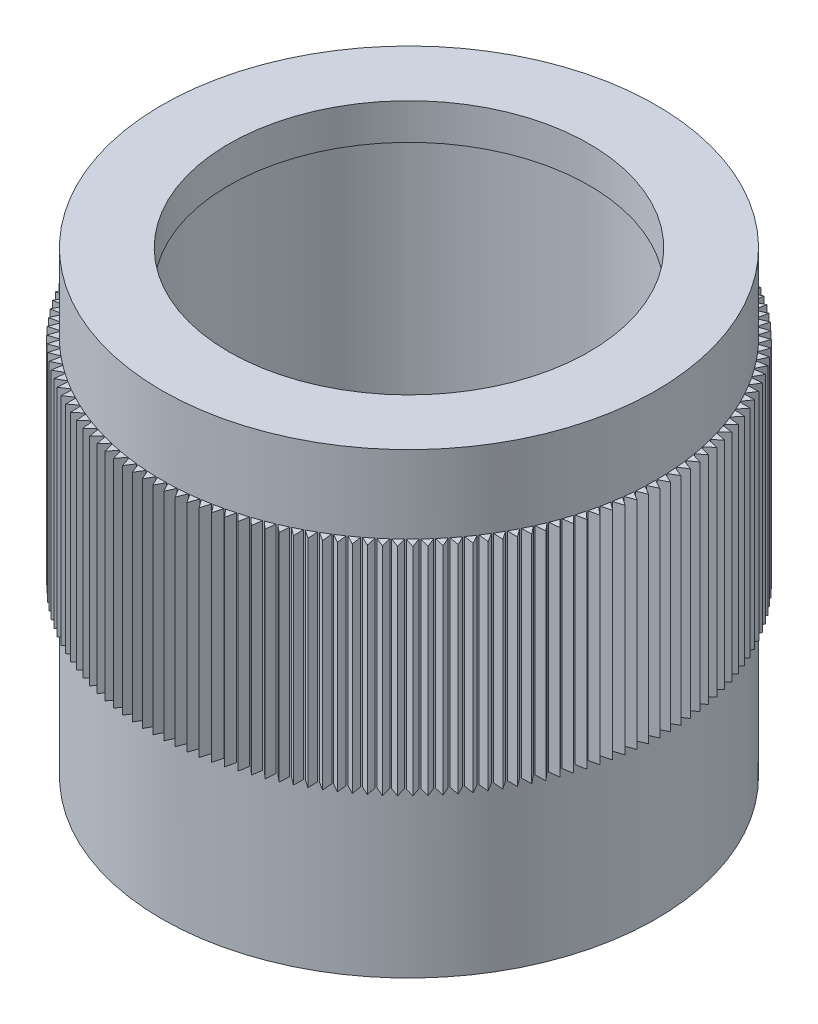
from build123d import *

# Parameters (mm, degrees)
BOSS_EXTRUDE1_DEPTH = 6
CHAMFER1_SIZE       = 0.5


with BuildPart() as part:
    # Sketch1 → Revolve1 (revolve)
    with BuildSketch(Plane.XY, mode=Mode.PRIVATE) as revolve1_sk:
        Polygon((-5, 11.7), (-5.25, 11.7), (-5.25, 0), (-6.86, 0), (-6.86, 12.7), (-5, 12.7), align=None)
    revolve(revolve1_sk.sketch.rotate(Axis((0, 15.254212557, 0), (0, -1, 0)), 270), axis=Axis((0, 15.254212557, 0), (0, -1, 0)))

    # Sketch2 → Boss-Extrude1 (add)
    with BuildSketch(Plane(origin=(0, 10.55, 0), x_dir=(-1, 0, 0), z_dir=(0, 1, 0))):
        with BuildLine():
            Line((-0.125, 6.858861057), (0, 7.11))
            Line((0, 7.11), (0.125, 6.858861057))
            ThreePointArc((0.125, 6.858861057), (0, 6.86), (-0.125, 6.858861057))
        make_face()
        with BuildLine():
            Line((0.162328937, 6.858079127), (0.297735898, 7.103763322))
            Line((0.297735898, 7.103763322), (0.412109644, 6.847610214))
            ThreePointArc((0.412109644, 6.847610214), (0.287266985, 6.853982614), (0.162328937, 6.858079127))
        make_face()
        with BuildLine():
            Line((0.449373094, 6.845265796), (0.594949466, 7.085064229))
            Line((0.594949466, 7.085064229), (0.698496308, 6.824346336))
            ThreePointArc((0.698496308, 6.824346336), (0.574030005, 6.835941014), (0.449373094, 6.845265796))
        make_face()
        with BuildLine():
            Line((0.735628897, 6.820443543), (0.891119291, 7.053935526))
            Line((0.891119291, 7.053935526), (0.983657573, 6.789110235))
            ThreePointArc((0.983657573, 6.789110235), (0.859785982, 6.805906851), (0.735628897, 6.820443543))
        make_face()
        with BuildLine():
            Line((1.020594158, 6.783655914), (1.185725789, 7.010431824))
            Line((1.185725789, 7.010431824), (1.267093167, 6.741963728))
            ThreePointArc((1.267093167, 6.741963728), (1.144033602, 6.763932814), (1.020594158, 6.783655914))
        make_face()
        with BuildLine():
            Line((1.303768949, 6.734967448), (1.478252122, 6.954629441))
            Line((1.478252122, 6.954629441), (1.54830585, 6.682989525))
            ThreePointArc((1.54830585, 6.682989525), (1.426274199, 6.710092541), (1.303768949, 6.734967448))
        make_face()
        with BuildLine():
            Line((1.584656487, 6.67446356), (1.768185098, 6.886626276))
            Line((1.768185098, 6.886626276), (1.826802277, 6.612291088))
            ThreePointArc((1.826802277, 6.612291088), (1.706012626, 6.644480485), (1.584656487, 6.67446356))
        make_face()
        with BuildLine():
            Line((1.862763999, 6.602250395), (2.055016076, 6.806541627))
            Line((2.055016076, 6.806541627), (2.102093874, 6.529992446))
            ThreePointArc((2.102093874, 6.529992446), (1.982758127, 6.567211753), (1.862763999, 6.602250395))
        make_face()
        with BuildLine():
            Line((2.13760359, 6.51845464), (2.338241858, 6.714515992))
            Line((2.338241858, 6.714515992), (2.373697683, 6.436237978))
            ThreePointArc((2.373697683, 6.436237978), (2.256025197, 6.4784219), (2.13760359, 6.51845464))
        make_face()
        with BuildLine():
            Line((2.408693098, 6.4232233), (2.61736557, 6.610710815))
            Line((2.61736557, 6.610710815), (2.641137219, 6.331192162))
            ThreePointArc((2.641137219, 6.331192162), (2.525334431, 6.378266693), (2.408693098, 6.4232233))
        make_face()
        with BuildLine():
            Line((2.675556939, 6.316723444), (2.891897532, 6.495308204))
            Line((2.891897532, 6.495308204), (2.903943304, 6.215039283))
            ThreePointArc((2.903943304, 6.215039283), (2.790213371, 6.266921839), (2.675556939, 6.316723444))
        make_face()
        with BuildLine():
            Line((2.937726945, 6.199141908), (3.161356124, 6.368510615))
            Line((3.161356124, 6.368510615), (3.161654885, 6.087983113))
            ThreePointArc((3.161654885, 6.087983113), (3.050197329, 6.144582675), (2.937726945, 6.199141908))
        make_face()
        with BuildLine():
            Line((3.194743179, 6.070684971), (3.425268623, 6.230540495))
            Line((3.425268623, 6.230540495), (3.413819849, 5.950246553))
            ThreePointArc((3.413819849, 5.950246553), (3.304830204, 6.011463825), (3.194743179, 6.070684971))
        make_face()
        with BuildLine():
            Line((3.446154749, 5.93157799), (3.683172037, 6.08163989))
            Line((3.683172037, 6.08163989), (3.659995814, 5.802071237))
            ThreePointArc((3.659995814, 5.802071237), (3.553665284, 5.867798825), (3.446154749, 5.93157799))
        make_face()
        with BuildLine():
            Line((3.691520591, 5.782065005), (3.934613915, 5.922070021))
            Line((3.934613915, 5.922070021), (3.899750901, 5.643717118))
            ThreePointArc((3.899750901, 5.643717118), (3.796266028, 5.713839711), (3.691520591, 5.782065005))
        make_face()
        with BuildLine():
            Line((3.930410253, 5.622408314), (4.179153144, 5.75211083))
            Line((4.179153144, 5.75211083), (4.132664501, 5.475462001))
            ThreePointArc((4.132664501, 5.475462001), (4.032206831, 5.549856581), (3.930410253, 5.622408314))
        make_face()
        with BuildLine():
            Line((4.162404639, 5.452888008), (4.416360718, 5.572060482))
            Line((4.416360718, 5.572060482), (4.358328003, 5.297601063))
            ThreePointArc((4.358328003, 5.297601063), (4.261073773, 5.376137117), (4.162404639, 5.452888008))
        make_face()
        with BuildLine():
            Line((4.387096753, 5.273801483), (4.645820494, 5.382234846))
            Line((4.645820494, 5.382234846), (4.576345517, 5.110446332))
            ThreePointArc((4.576345517, 5.110446332), (4.482465343, 5.192986082), (4.387096753, 5.273801483))
        make_face()
        with BuildLine():
            Line((4.604092408, 5.085462919), (4.867129923, 5.182966941))
            Line((4.867129923, 5.182966941), (4.786334565, 4.914326142))
            ThreePointArc((4.786334565, 4.914326142), (4.695993147, 5.000724784), (4.604092408, 5.085462919))
        make_face()
        with BuildLine():
            Line((4.813010921, 4.888202724), (5.079900752, 4.974606351))
            Line((5.079900752, 4.974606351), (4.987926756, 4.709584554))
            ThreePointArc((4.987926756, 4.709584554), (4.901282582, 4.799690516), (4.813010921, 4.888202724))
        make_face()
        with BuildLine():
            Line((5.013485777, 4.682366961), (5.283759709, 4.757518611))
            Line((5.283759709, 4.757518611), (5.180768429, 4.496580755))
            ThreePointArc((5.180768429, 4.496580755), (5.097973503, 4.59023596), (5.013485777, 4.682366961))
        make_face()
        with BuildLine():
            Line((5.205165276, 4.468316735), (5.478349156, 4.532084567))
            Line((5.478349156, 4.532084567), (5.364521274, 4.275688425))
            ThreePointArc((5.364521274, 4.275688425), (5.285720845, 4.37272857), (5.205165276, 4.468316735))
        make_face()
        with BuildLine():
            Line((5.387713146, 4.246427564), (5.663327717, 4.298699707))
            Line((5.663327717, 4.298699707), (5.538862925, 4.047295084))
            ThreePointArc((5.538862925, 4.047295084), (5.464195238, 4.147549928), (5.387713146, 4.246427564))
        make_face()
        with BuildLine():
            Line((5.560809137, 4.017088715), (5.838370877, 4.057773466))
            Line((5.838370877, 4.057773466), (5.703487529, 3.811801413))
            ThreePointArc((5.703487529, 3.811801413), (5.633083575, 3.915095074), (5.560809137, 4.017088715))
        make_face()
        with BuildLine():
            Line((5.724149578, 3.780702528), (6.00317155, 3.809728512))
            Line((6.00317155, 3.809728512), (5.858106277, 3.569620547))
            ThreePointArc((5.858106277, 3.569620547), (5.792089569, 3.675771814), (5.724149578, 3.780702528))
        make_face()
        with BuildLine():
            Line((5.877447916, 3.537683704), (6.157440621, 3.555))
            Line((6.157440621, 3.555), (6.002447916, 3.321177353))
            ThreePointArc((6.002447916, 3.321177353), (5.94093427, 3.43), (5.877447916, 3.537683704))
        make_face()
        with BuildLine():
            Line((6.020435214, 3.288458581), (6.300907448, 3.29403481))
            Line((6.300907448, 3.29403481), (6.136259223, 3.066907686))
            ThreePointArc((6.136259223, 3.066907686), (6.079356554, 3.178210801), (6.020435214, 3.288458581))
        make_face()
        with BuildLine():
            Line((6.152860622, 3.033464383), (6.433320343, 3.027290763))
            Line((6.433320343, 3.027290763), (6.259305445, 2.80725762))
            ThreePointArc((6.259305445, 2.80725762), (6.20711358, 2.92084594), (6.152860622, 3.033464383))
        make_face()
        with BuildLine():
            Line((6.274491822, 2.773148459), (6.554447008, 2.75523582))
            Line((6.554447008, 2.75523582), (6.371370719, 2.542682671))
            ThreePointArc((6.371370719, 2.542682671), (6.32398122, 2.658356923), (6.274491822, 2.773148459))
        make_face()
        with BuildLine():
            Line((6.385115431, 2.50796749), (6.664074945, 2.478347256))
            Line((6.664074945, 2.478347256), (6.472258443, 2.273646992))
            ThreePointArc((6.472258443, 2.273646992), (6.429754448, 2.391204245), (6.385115431, 2.50796749))
        make_face()
        with BuildLine():
            Line((6.484537378, 2.238386693), (6.762011831, 2.19711083))
            Line((6.762011831, 2.19711083), (6.561791627, 2.000622564))
            ThreePointArc((6.561791627, 2.000622564), (6.524247702, 2.119856581), (6.484537378, 2.238386693))
        make_face()
        with BuildLine():
            Line((6.572583243, 1.964879006), (6.84808585, 1.912019925))
            Line((6.84808585, 1.912019925), (6.639813199, 1.724088364))
            ThreePointArc((6.639813199, 1.724088364), (6.607295208, 1.844789969), (6.572583243, 1.964879006))
        make_face()
        with BuildLine():
            Line((6.649098564, 1.687924253), (6.922145999, 1.623574686))
            Line((6.922145999, 1.623574686), (6.706186282, 1.444529527))
            ThreePointArc((6.706186282, 1.444529527), (6.678751274, 1.566486969), (6.649098564, 1.687924253))
        make_face()
        with BuildLine():
            Line((6.713949107, 1.408008308), (6.984062353, 1.332281147))
            Line((6.984062353, 1.332281147), (6.760794435, 1.162436495))
            ThreePointArc((6.760794435, 1.162436495), (6.73849054, 1.285435818), (6.713949107, 1.408008308))
        make_face()
        with BuildLine():
            Line((6.767021101, 1.125622237), (7.033726287, 1.038650333))
            Line((7.033726287, 1.038650333), (6.803541858, 0.878304154))
            ThreePointArc((6.803541858, 0.878304154), (6.786408204, 1.002129576), (6.767021101, 1.125622237))
        make_face()
        with BuildLine():
            Line((6.808221441, 0.841261443), (7.071050676, 0.743197374))
            Line((7.071050676, 0.743197374), (6.834353556, 0.592630969))
            ThreePointArc((6.834353556, 0.592630969), (6.822420202, 0.717065258), (6.808221441, 0.841261443))
        make_face()
        with BuildLine():
            Line((6.837477847, 0.55542479), (7.095970039, 0.446440594))
            Line((7.095970039, 0.446440594), (6.853175476, 0.305918108))
            ThreePointArc((6.853175476, 0.305918108), (6.846463357, 0.430742964), (6.837477847, 0.55542479))
        make_face()
        with BuildLine():
            Line((6.854738993, 0.268613734), (7.10844066, 0.148900605))
            Line((7.10844066, 0.148900605), (6.859974598, 0.018668563))
            ThreePointArc((6.859974598, 0.018668563), (6.858495489, 0.143665), (6.854738993, 0.268613734))
        make_face()
        with BuildLine():
            Line((6.859974598, -0.018668563), (7.10844066, -0.148900605))
            Line((7.10844066, -0.148900605), (6.854738993, -0.268613734))
            ThreePointArc((6.854738993, -0.268613734), (6.858495489, -0.143665), (6.859974598, -0.018668563))
        make_face()
        with BuildLine():
            Line((6.853175476, -0.305918108), (7.095970039, -0.446440594))
            Line((7.095970039, -0.446440594), (6.837477847, -0.55542479))
            ThreePointArc((6.837477847, -0.55542479), (6.846463357, -0.430742964), (6.853175476, -0.305918108))
        make_face()
        with BuildLine():
            Line((6.834353556, -0.592630969), (7.071050676, -0.743197374))
            Line((7.071050676, -0.743197374), (6.808221441, -0.841261443))
            ThreePointArc((6.808221441, -0.841261443), (6.822420202, -0.717065258), (6.834353556, -0.592630969))
        make_face()
        with BuildLine():
            Line((6.803541858, -0.878304154), (7.033726287, -1.038650333))
            Line((7.033726287, -1.038650333), (6.767021101, -1.125622237))
            ThreePointArc((6.767021101, -1.125622237), (6.786408204, -1.002129576), (6.803541858, -0.878304154))
        make_face()
        with BuildLine():
            Line((6.760794435, -1.162436495), (6.984062353, -1.332281147))
            Line((6.984062353, -1.332281147), (6.713949107, -1.408008308))
            ThreePointArc((6.713949107, -1.408008308), (6.73849054, -1.285435818), (6.760794435, -1.162436495))
        make_face()
        with BuildLine():
            Line((6.706186282, -1.444529527), (6.922145999, -1.623574686))
            Line((6.922145999, -1.623574686), (6.649098564, -1.687924253))
            ThreePointArc((6.649098564, -1.687924253), (6.678751274, -1.566486969), (6.706186282, -1.444529527))
        make_face()
        with BuildLine():
            Line((6.639813199, -1.724088364), (6.84808585, -1.912019925))
            Line((6.84808585, -1.912019925), (6.572583243, -1.964879006))
            ThreePointArc((6.572583243, -1.964879006), (6.607295208, -1.844789969), (6.639813199, -1.724088364))
        make_face()
        with BuildLine():
            Line((6.561791627, -2.000622564), (6.762011831, -2.19711083))
            Line((6.762011831, -2.19711083), (6.484537378, -2.238386693))
            ThreePointArc((6.484537378, -2.238386693), (6.524247702, -2.119856581), (6.561791627, -2.000622564))
        make_face()
        with BuildLine():
            Line((6.472258443, -2.273646992), (6.664074945, -2.478347256))
            Line((6.664074945, -2.478347256), (6.385115431, -2.50796749))
            ThreePointArc((6.385115431, -2.50796749), (6.429754448, -2.391204245), (6.472258443, -2.273646992))
        make_face()
        with BuildLine():
            Line((6.371370719, -2.542682671), (6.554447008, -2.75523582))
            Line((6.554447008, -2.75523582), (6.274491822, -2.773148459))
            ThreePointArc((6.274491822, -2.773148459), (6.32398122, -2.658356923), (6.371370719, -2.542682671))
        make_face()
        with BuildLine():
            Line((6.259305445, -2.80725762), (6.433320343, -3.027290763))
            Line((6.433320343, -3.027290763), (6.152860622, -3.033464383))
            ThreePointArc((6.152860622, -3.033464383), (6.20711358, -2.92084594), (6.259305445, -2.80725762))
        make_face()
        with BuildLine():
            Line((6.136259223, -3.066907686), (6.300907448, -3.29403481))
            Line((6.300907448, -3.29403481), (6.020435214, -3.288458581))
            ThreePointArc((6.020435214, -3.288458581), (6.079356554, -3.178210801), (6.136259223, -3.066907686))
        make_face()
        with BuildLine():
            Line((6.002447916, -3.321177353), (6.157440621, -3.555))
            Line((6.157440621, -3.555), (5.877447916, -3.537683704))
            ThreePointArc((5.877447916, -3.537683704), (5.94093427, -3.43), (6.002447916, -3.321177353))
        make_face()
        with BuildLine():
            Line((5.858106277, -3.569620547), (6.00317155, -3.809728512))
            Line((6.00317155, -3.809728512), (5.724149578, -3.780702528))
            ThreePointArc((5.724149578, -3.780702528), (5.792089569, -3.675771814), (5.858106277, -3.569620547))
        make_face()
        with BuildLine():
            Line((5.703487529, -3.811801413), (5.838370877, -4.057773466))
            Line((5.838370877, -4.057773466), (5.560809137, -4.017088715))
            ThreePointArc((5.560809137, -4.017088715), (5.633083575, -3.915095074), (5.703487529, -3.811801413))
        make_face()
        with BuildLine():
            Line((5.538862925, -4.047295084), (5.663327717, -4.298699707))
            Line((5.663327717, -4.298699707), (5.387713146, -4.246427564))
            ThreePointArc((5.387713146, -4.246427564), (5.464195238, -4.147549928), (5.538862925, -4.047295084))
        make_face()
        with BuildLine():
            Line((5.364521274, -4.275688425), (5.478349156, -4.532084567))
            Line((5.478349156, -4.532084567), (5.205165276, -4.468316735))
            ThreePointArc((5.205165276, -4.468316735), (5.285720845, -4.37272857), (5.364521274, -4.275688425))
        make_face()
        with BuildLine():
            Line((5.180768429, -4.496580755), (5.283759709, -4.757518611))
            Line((5.283759709, -4.757518611), (5.013485777, -4.682366961))
            ThreePointArc((5.013485777, -4.682366961), (5.097973503, -4.59023596), (5.180768429, -4.496580755))
        make_face()
        with BuildLine():
            Line((4.987926756, -4.709584554), (5.079900752, -4.974606351))
            Line((5.079900752, -4.974606351), (4.813010921, -4.888202724))
            ThreePointArc((4.813010921, -4.888202724), (4.901282582, -4.799690516), (4.987926756, -4.709584554))
        make_face()
        with BuildLine():
            Line((4.786334565, -4.914326142), (4.867129923, -5.182966941))
            Line((4.867129923, -5.182966941), (4.604092408, -5.085462919))
            ThreePointArc((4.604092408, -5.085462919), (4.695993147, -5.000724784), (4.786334565, -4.914326142))
        make_face()
        with BuildLine():
            Line((4.576345517, -5.110446332), (4.645820494, -5.382234846))
            Line((4.645820494, -5.382234846), (4.387096753, -5.273801483))
            ThreePointArc((4.387096753, -5.273801483), (4.482465343, -5.192986082), (4.576345517, -5.110446332))
        make_face()
        with BuildLine():
            Line((4.358328003, -5.297601063), (4.416360718, -5.572060482))
            Line((4.416360718, -5.572060482), (4.162404639, -5.452888008))
            ThreePointArc((4.162404639, -5.452888008), (4.261073773, -5.376137117), (4.358328003, -5.297601063))
        make_face()
        with BuildLine():
            Line((4.132664501, -5.475462001), (4.179153144, -5.75211083))
            Line((4.179153144, -5.75211083), (3.930410253, -5.622408314))
            ThreePointArc((3.930410253, -5.622408314), (4.032206831, -5.549856581), (4.132664501, -5.475462001))
        make_face()
        with BuildLine():
            Line((3.899750901, -5.643717118), (3.934613915, -5.922070021))
            Line((3.934613915, -5.922070021), (3.691520591, -5.782065005))
            ThreePointArc((3.691520591, -5.782065005), (3.796266028, -5.713839711), (3.899750901, -5.643717118))
        make_face()
        with BuildLine():
            Line((3.659995814, -5.802071237), (3.683172037, -6.08163989))
            Line((3.683172037, -6.08163989), (3.446154749, -5.93157799))
            ThreePointArc((3.446154749, -5.93157799), (3.553665284, -5.867798825), (3.659995814, -5.802071237))
        make_face()
        with BuildLine():
            Line((3.413819849, -5.950246553), (3.425268623, -6.230540495))
            Line((3.425268623, -6.230540495), (3.194743179, -6.070684971))
            ThreePointArc((3.194743179, -6.070684971), (3.304830204, -6.011463825), (3.413819849, -5.950246553))
        make_face()
        with BuildLine():
            Line((3.161654885, -6.087983113), (3.161356124, -6.368510615))
            Line((3.161356124, -6.368510615), (2.937726945, -6.199141908))
            ThreePointArc((2.937726945, -6.199141908), (3.050197329, -6.144582675), (3.161654885, -6.087983113))
        make_face()
        with BuildLine():
            Line((2.903943304, -6.215039283), (2.891897532, -6.495308204))
            Line((2.891897532, -6.495308204), (2.675556939, -6.316723444))
            ThreePointArc((2.675556939, -6.316723444), (2.790213372, -6.266921839), (2.903943304, -6.215039283))
        make_face()
        with BuildLine():
            Line((2.641137219, -6.331192162), (2.61736557, -6.610710815))
            Line((2.61736557, -6.610710815), (2.408693098, -6.4232233))
            ThreePointArc((2.408693098, -6.4232233), (2.525334431, -6.378266693), (2.641137219, -6.331192162))
        make_face()
        with BuildLine():
            Line((2.373697683, -6.436237978), (2.338241858, -6.714515992))
            Line((2.338241858, -6.714515992), (2.13760359, -6.51845464))
            ThreePointArc((2.13760359, -6.51845464), (2.256025197, -6.4784219), (2.373697683, -6.436237978))
        make_face()
        with BuildLine():
            Line((2.102093874, -6.529992446), (2.055016076, -6.806541627))
            Line((2.055016076, -6.806541627), (1.862763999, -6.602250395))
            ThreePointArc((1.862763999, -6.602250395), (1.982758127, -6.567211753), (2.102093874, -6.529992446))
        make_face()
        with BuildLine():
            Line((1.826802277, -6.612291088), (1.768185098, -6.886626276))
            Line((1.768185098, -6.886626276), (1.584656487, -6.67446356))
            ThreePointArc((1.584656487, -6.67446356), (1.706012626, -6.644480485), (1.826802277, -6.612291088))
        make_face()
        with BuildLine():
            Line((1.54830585, -6.682989525), (1.478252122, -6.954629441))
            Line((1.478252122, -6.954629441), (1.303768949, -6.734967448))
            ThreePointArc((1.303768949, -6.734967448), (1.426274199, -6.710092541), (1.54830585, -6.682989525))
        make_face()
        with BuildLine():
            Line((1.267093167, -6.741963728), (1.185725789, -7.010431824))
            Line((1.185725789, -7.010431824), (1.020594158, -6.783655914))
            ThreePointArc((1.020594158, -6.783655914), (1.144033602, -6.763932814), (1.267093167, -6.741963728))
        make_face()
        with BuildLine():
            Line((0.983657573, -6.789110235), (0.891119291, -7.053935526))
            Line((0.891119291, -7.053935526), (0.735628897, -6.820443543))
            ThreePointArc((0.735628897, -6.820443543), (0.859785982, -6.805906851), (0.983657573, -6.789110235))
        make_face()
        with BuildLine():
            Line((0.698496308, -6.824346336), (0.594949466, -7.085064229))
            Line((0.594949466, -7.085064229), (0.449373094, -6.845265796))
            ThreePointArc((0.449373094, -6.845265796), (0.574030005, -6.835941014), (0.698496308, -6.824346336))
        make_face()
        with BuildLine():
            Line((0.412109644, -6.847610214), (0.297735898, -7.103763322))
            Line((0.297735898, -7.103763322), (0.162328937, -6.858079127))
            ThreePointArc((0.162328937, -6.858079127), (0.287266985, -6.853982614), (0.412109644, -6.847610214))
        make_face()
        with BuildLine():
            Line((0.125, -6.858861057), (0, -7.11))
            Line((0, -7.11), (-0.125, -6.858861057))
            ThreePointArc((-0.125, -6.858861057), (0, -6.86), (0.125, -6.858861057))
        make_face()
        with BuildLine():
            Line((-0.162328937, -6.858079127), (-0.297735898, -7.103763322))
            Line((-0.297735898, -7.103763322), (-0.412109644, -6.847610214))
            ThreePointArc((-0.412109644, -6.847610214), (-0.287266985, -6.853982614), (-0.162328937, -6.858079127))
        make_face()
        with BuildLine():
            Line((-0.449373094, -6.845265796), (-0.594949466, -7.085064229))
            Line((-0.594949466, -7.085064229), (-0.698496308, -6.824346336))
            ThreePointArc((-0.698496308, -6.824346336), (-0.574030005, -6.835941014), (-0.449373094, -6.845265796))
        make_face()
        with BuildLine():
            Line((-0.735628897, -6.820443543), (-0.891119291, -7.053935526))
            Line((-0.891119291, -7.053935526), (-0.983657573, -6.789110235))
            ThreePointArc((-0.983657573, -6.789110235), (-0.859785982, -6.805906851), (-0.735628897, -6.820443543))
        make_face()
        with BuildLine():
            Line((-1.020594158, -6.783655914), (-1.185725789, -7.010431824))
            Line((-1.185725789, -7.010431824), (-1.267093167, -6.741963728))
            ThreePointArc((-1.267093167, -6.741963728), (-1.144033602, -6.763932814), (-1.020594158, -6.783655914))
        make_face()
        with BuildLine():
            Line((-1.303768949, -6.734967448), (-1.478252122, -6.954629441))
            Line((-1.478252122, -6.954629441), (-1.54830585, -6.682989525))
            ThreePointArc((-1.54830585, -6.682989525), (-1.426274199, -6.710092541), (-1.303768949, -6.734967448))
        make_face()
        with BuildLine():
            Line((-1.584656487, -6.67446356), (-1.768185098, -6.886626276))
            Line((-1.768185098, -6.886626276), (-1.826802277, -6.612291088))
            ThreePointArc((-1.826802277, -6.612291088), (-1.706012626, -6.644480485), (-1.584656487, -6.67446356))
        make_face()
        with BuildLine():
            Line((-1.862763999, -6.602250395), (-2.055016076, -6.806541627))
            Line((-2.055016076, -6.806541627), (-2.102093874, -6.529992446))
            ThreePointArc((-2.102093874, -6.529992446), (-1.982758127, -6.567211753), (-1.862763999, -6.602250395))
        make_face()
        with BuildLine():
            Line((-2.13760359, -6.51845464), (-2.338241858, -6.714515992))
            Line((-2.338241858, -6.714515992), (-2.373697683, -6.436237978))
            ThreePointArc((-2.373697683, -6.436237978), (-2.256025197, -6.4784219), (-2.13760359, -6.51845464))
        make_face()
        with BuildLine():
            Line((-2.408693098, -6.4232233), (-2.61736557, -6.610710815))
            Line((-2.61736557, -6.610710815), (-2.641137219, -6.331192162))
            ThreePointArc((-2.641137219, -6.331192162), (-2.525334431, -6.378266693), (-2.408693098, -6.4232233))
        make_face()
        with BuildLine():
            Line((-2.675556939, -6.316723444), (-2.891897532, -6.495308204))
            Line((-2.891897532, -6.495308204), (-2.903943304, -6.215039283))
            ThreePointArc((-2.903943304, -6.215039283), (-2.790213371, -6.266921839), (-2.675556939, -6.316723444))
        make_face()
        with BuildLine():
            Line((-2.937726945, -6.199141908), (-3.161356124, -6.368510615))
            Line((-3.161356124, -6.368510615), (-3.161654885, -6.087983113))
            ThreePointArc((-3.161654885, -6.087983113), (-3.050197329, -6.144582675), (-2.937726945, -6.199141908))
        make_face()
        with BuildLine():
            Line((-3.194743179, -6.070684971), (-3.425268623, -6.230540495))
            Line((-3.425268623, -6.230540495), (-3.413819849, -5.950246553))
            ThreePointArc((-3.413819849, -5.950246553), (-3.304830204, -6.011463825), (-3.194743179, -6.070684971))
        make_face()
        with BuildLine():
            Line((-3.446154749, -5.93157799), (-3.683172037, -6.08163989))
            Line((-3.683172037, -6.08163989), (-3.659995814, -5.802071237))
            ThreePointArc((-3.659995814, -5.802071237), (-3.553665284, -5.867798825), (-3.446154749, -5.93157799))
        make_face()
        with BuildLine():
            Line((-3.691520591, -5.782065005), (-3.934613915, -5.922070021))
            Line((-3.934613915, -5.922070021), (-3.899750901, -5.643717118))
            ThreePointArc((-3.899750901, -5.643717118), (-3.796266028, -5.713839711), (-3.691520591, -5.782065005))
        make_face()
        with BuildLine():
            Line((-3.930410253, -5.622408314), (-4.179153144, -5.75211083))
            Line((-4.179153144, -5.75211083), (-4.132664501, -5.475462001))
            ThreePointArc((-4.132664501, -5.475462001), (-4.032206831, -5.549856581), (-3.930410253, -5.622408314))
        make_face()
        with BuildLine():
            Line((-4.162404639, -5.452888008), (-4.416360718, -5.572060482))
            Line((-4.416360718, -5.572060482), (-4.358328003, -5.297601063))
            ThreePointArc((-4.358328003, -5.297601063), (-4.261073773, -5.376137117), (-4.162404639, -5.452888008))
        make_face()
        with BuildLine():
            Line((-4.387096753, -5.273801483), (-4.645820494, -5.382234846))
            Line((-4.645820494, -5.382234846), (-4.576345517, -5.110446332))
            ThreePointArc((-4.576345517, -5.110446332), (-4.482465343, -5.192986082), (-4.387096753, -5.273801483))
        make_face()
        with BuildLine():
            Line((-4.604092408, -5.085462919), (-4.867129923, -5.182966941))
            Line((-4.867129923, -5.182966941), (-4.786334565, -4.914326142))
            ThreePointArc((-4.786334565, -4.914326142), (-4.695993147, -5.000724784), (-4.604092408, -5.085462919))
        make_face()
        with BuildLine():
            Line((-4.813010921, -4.888202724), (-5.079900752, -4.974606351))
            Line((-5.079900752, -4.974606351), (-4.987926756, -4.709584554))
            ThreePointArc((-4.987926756, -4.709584554), (-4.901282582, -4.799690516), (-4.813010921, -4.888202724))
        make_face()
        with BuildLine():
            Line((-5.013485777, -4.682366961), (-5.283759709, -4.757518611))
            Line((-5.283759709, -4.757518611), (-5.180768429, -4.496580755))
            ThreePointArc((-5.180768429, -4.496580755), (-5.097973503, -4.59023596), (-5.013485777, -4.682366961))
        make_face()
        with BuildLine():
            Line((-5.205165276, -4.468316735), (-5.478349156, -4.532084567))
            Line((-5.478349156, -4.532084567), (-5.364521274, -4.275688425))
            ThreePointArc((-5.364521274, -4.275688425), (-5.285720845, -4.37272857), (-5.205165276, -4.468316735))
        make_face()
        with BuildLine():
            Line((-5.387713146, -4.246427564), (-5.663327717, -4.298699707))
            Line((-5.663327717, -4.298699707), (-5.538862925, -4.047295084))
            ThreePointArc((-5.538862925, -4.047295084), (-5.464195238, -4.147549928), (-5.387713146, -4.246427564))
        make_face()
        with BuildLine():
            Line((-5.560809137, -4.017088715), (-5.838370877, -4.057773466))
            Line((-5.838370877, -4.057773466), (-5.703487529, -3.811801413))
            ThreePointArc((-5.703487529, -3.811801413), (-5.633083575, -3.915095074), (-5.560809137, -4.017088715))
        make_face()
        with BuildLine():
            Line((-5.724149578, -3.780702528), (-6.00317155, -3.809728512))
            Line((-6.00317155, -3.809728512), (-5.858106277, -3.569620547))
            ThreePointArc((-5.858106277, -3.569620547), (-5.792089569, -3.675771814), (-5.724149578, -3.780702528))
        make_face()
        with BuildLine():
            Line((-5.877447916, -3.537683704), (-6.157440621, -3.555))
            Line((-6.157440621, -3.555), (-6.002447916, -3.321177353))
            ThreePointArc((-6.002447916, -3.321177353), (-5.94093427, -3.43), (-5.877447916, -3.537683704))
        make_face()
        with BuildLine():
            Line((-6.020435214, -3.288458581), (-6.300907448, -3.29403481))
            Line((-6.300907448, -3.29403481), (-6.136259223, -3.066907686))
            ThreePointArc((-6.136259223, -3.066907686), (-6.079356554, -3.178210801), (-6.020435214, -3.288458581))
        make_face()
        with BuildLine():
            Line((-6.152860622, -3.033464383), (-6.433320343, -3.027290763))
            Line((-6.433320343, -3.027290763), (-6.259305445, -2.80725762))
            ThreePointArc((-6.259305445, -2.80725762), (-6.20711358, -2.92084594), (-6.152860622, -3.033464383))
        make_face()
        with BuildLine():
            Line((-6.274491822, -2.773148459), (-6.554447008, -2.75523582))
            Line((-6.554447008, -2.75523582), (-6.371370719, -2.542682671))
            ThreePointArc((-6.371370719, -2.542682671), (-6.32398122, -2.658356923), (-6.274491822, -2.773148459))
        make_face()
        with BuildLine():
            Line((-6.385115431, -2.50796749), (-6.664074945, -2.478347256))
            Line((-6.664074945, -2.478347256), (-6.472258443, -2.273646992))
            ThreePointArc((-6.472258443, -2.273646992), (-6.429754448, -2.391204245), (-6.385115431, -2.50796749))
        make_face()
        with BuildLine():
            Line((-6.484537378, -2.238386693), (-6.762011831, -2.19711083))
            Line((-6.762011831, -2.19711083), (-6.561791627, -2.000622564))
            ThreePointArc((-6.561791627, -2.000622564), (-6.524247702, -2.119856581), (-6.484537378, -2.238386693))
        make_face()
        with BuildLine():
            Line((-6.572583243, -1.964879006), (-6.84808585, -1.912019925))
            Line((-6.84808585, -1.912019925), (-6.639813199, -1.724088364))
            ThreePointArc((-6.639813199, -1.724088364), (-6.607295208, -1.844789969), (-6.572583243, -1.964879006))
        make_face()
        with BuildLine():
            Line((-6.649098564, -1.687924253), (-6.922145999, -1.623574686))
            Line((-6.922145999, -1.623574686), (-6.706186282, -1.444529527))
            ThreePointArc((-6.706186282, -1.444529527), (-6.678751274, -1.566486969), (-6.649098564, -1.687924253))
        make_face()
        with BuildLine():
            Line((-6.713949107, -1.408008308), (-6.984062353, -1.332281147))
            Line((-6.984062353, -1.332281147), (-6.760794435, -1.162436495))
            ThreePointArc((-6.760794435, -1.162436495), (-6.73849054, -1.285435818), (-6.713949107, -1.408008308))
        make_face()
        with BuildLine():
            Line((-6.767021101, -1.125622237), (-7.033726287, -1.038650333))
            Line((-7.033726287, -1.038650333), (-6.803541858, -0.878304154))
            ThreePointArc((-6.803541858, -0.878304154), (-6.786408204, -1.002129576), (-6.767021101, -1.125622237))
        make_face()
        with BuildLine():
            Line((-6.808221441, -0.841261443), (-7.071050676, -0.743197374))
            Line((-7.071050676, -0.743197374), (-6.834353556, -0.592630969))
            ThreePointArc((-6.834353556, -0.592630969), (-6.822420202, -0.717065258), (-6.808221441, -0.841261443))
        make_face()
        with BuildLine():
            Line((-6.837477847, -0.55542479), (-7.095970039, -0.446440594))
            Line((-7.095970039, -0.446440594), (-6.853175476, -0.305918108))
            ThreePointArc((-6.853175476, -0.305918108), (-6.846463357, -0.430742964), (-6.837477847, -0.55542479))
        make_face()
        with BuildLine():
            Line((-6.854738993, -0.268613734), (-7.10844066, -0.148900605))
            Line((-7.10844066, -0.148900605), (-6.859974598, -0.018668563))
            ThreePointArc((-6.859974598, -0.018668563), (-6.858495489, -0.143665), (-6.854738993, -0.268613734))
        make_face()
        with BuildLine():
            Line((-6.859974598, 0.018668563), (-7.10844066, 0.148900605))
            Line((-7.10844066, 0.148900605), (-6.854738993, 0.268613734))
            ThreePointArc((-6.854738993, 0.268613734), (-6.858495489, 0.143665), (-6.859974598, 0.018668563))
        make_face()
        with BuildLine():
            Line((-6.853175476, 0.305918108), (-7.095970039, 0.446440594))
            Line((-7.095970039, 0.446440594), (-6.837477847, 0.55542479))
            ThreePointArc((-6.837477847, 0.55542479), (-6.846463357, 0.430742964), (-6.853175476, 0.305918108))
        make_face()
        with BuildLine():
            Line((-6.834353556, 0.592630969), (-7.071050676, 0.743197374))
            Line((-7.071050676, 0.743197374), (-6.808221441, 0.841261443))
            ThreePointArc((-6.808221441, 0.841261443), (-6.822420202, 0.717065258), (-6.834353556, 0.592630969))
        make_face()
        with BuildLine():
            Line((-6.803541858, 0.878304154), (-7.033726287, 1.038650333))
            Line((-7.033726287, 1.038650333), (-6.767021101, 1.125622237))
            ThreePointArc((-6.767021101, 1.125622237), (-6.786408204, 1.002129576), (-6.803541858, 0.878304154))
        make_face()
        with BuildLine():
            Line((-6.760794435, 1.162436495), (-6.984062353, 1.332281147))
            Line((-6.984062353, 1.332281147), (-6.713949107, 1.408008308))
            ThreePointArc((-6.713949107, 1.408008308), (-6.73849054, 1.285435818), (-6.760794435, 1.162436495))
        make_face()
        with BuildLine():
            Line((-6.706186282, 1.444529527), (-6.922145999, 1.623574686))
            Line((-6.922145999, 1.623574686), (-6.649098564, 1.687924253))
            ThreePointArc((-6.649098564, 1.687924253), (-6.678751274, 1.566486969), (-6.706186282, 1.444529527))
        make_face()
        with BuildLine():
            Line((-6.639813199, 1.724088364), (-6.84808585, 1.912019925))
            Line((-6.84808585, 1.912019925), (-6.572583243, 1.964879006))
            ThreePointArc((-6.572583243, 1.964879006), (-6.607295208, 1.844789969), (-6.639813199, 1.724088364))
        make_face()
        with BuildLine():
            Line((-6.561791627, 2.000622564), (-6.762011831, 2.19711083))
            Line((-6.762011831, 2.19711083), (-6.484537378, 2.238386693))
            ThreePointArc((-6.484537378, 2.238386693), (-6.524247702, 2.119856581), (-6.561791627, 2.000622564))
        make_face()
        with BuildLine():
            Line((-6.472258443, 2.273646992), (-6.664074945, 2.478347256))
            Line((-6.664074945, 2.478347256), (-6.385115431, 2.50796749))
            ThreePointArc((-6.385115431, 2.50796749), (-6.429754448, 2.391204245), (-6.472258443, 2.273646992))
        make_face()
        with BuildLine():
            Line((-6.371370719, 2.542682671), (-6.554447008, 2.75523582))
            Line((-6.554447008, 2.75523582), (-6.274491822, 2.773148459))
            ThreePointArc((-6.274491822, 2.773148459), (-6.32398122, 2.658356923), (-6.371370719, 2.542682671))
        make_face()
        with BuildLine():
            Line((-6.259305445, 2.80725762), (-6.433320343, 3.027290763))
            Line((-6.433320343, 3.027290763), (-6.152860622, 3.033464383))
            ThreePointArc((-6.152860622, 3.033464383), (-6.20711358, 2.92084594), (-6.259305445, 2.80725762))
        make_face()
        with BuildLine():
            Line((-6.136259223, 3.066907686), (-6.300907448, 3.29403481))
            Line((-6.300907448, 3.29403481), (-6.020435214, 3.288458581))
            ThreePointArc((-6.020435214, 3.288458581), (-6.079356554, 3.178210801), (-6.136259223, 3.066907686))
        make_face()
        with BuildLine():
            Line((-6.002447916, 3.321177353), (-6.157440621, 3.555))
            Line((-6.157440621, 3.555), (-5.877447916, 3.537683704))
            ThreePointArc((-5.877447916, 3.537683704), (-5.94093427, 3.43), (-6.002447916, 3.321177353))
        make_face()
        with BuildLine():
            Line((-5.858106277, 3.569620547), (-6.00317155, 3.809728512))
            Line((-6.00317155, 3.809728512), (-5.724149578, 3.780702528))
            ThreePointArc((-5.724149578, 3.780702528), (-5.792089569, 3.675771814), (-5.858106277, 3.569620547))
        make_face()
        with BuildLine():
            Line((-5.703487529, 3.811801413), (-5.838370877, 4.057773466))
            Line((-5.838370877, 4.057773466), (-5.560809137, 4.017088715))
            ThreePointArc((-5.560809137, 4.017088715), (-5.633083575, 3.915095074), (-5.703487529, 3.811801413))
        make_face()
        with BuildLine():
            Line((-5.538862925, 4.047295084), (-5.663327717, 4.298699707))
            Line((-5.663327717, 4.298699707), (-5.387713146, 4.246427564))
            ThreePointArc((-5.387713146, 4.246427564), (-5.464195238, 4.147549928), (-5.538862925, 4.047295084))
        make_face()
        with BuildLine():
            Line((-5.364521274, 4.275688425), (-5.478349156, 4.532084567))
            Line((-5.478349156, 4.532084567), (-5.205165276, 4.468316735))
            ThreePointArc((-5.205165276, 4.468316735), (-5.285720845, 4.37272857), (-5.364521274, 4.275688425))
        make_face()
        with BuildLine():
            Line((-5.180768429, 4.496580755), (-5.283759709, 4.757518611))
            Line((-5.283759709, 4.757518611), (-5.013485777, 4.682366961))
            ThreePointArc((-5.013485777, 4.682366961), (-5.097973503, 4.59023596), (-5.180768429, 4.496580755))
        make_face()
        with BuildLine():
            Line((-4.987926756, 4.709584554), (-5.079900752, 4.974606351))
            Line((-5.079900752, 4.974606351), (-4.813010921, 4.888202724))
            ThreePointArc((-4.813010921, 4.888202724), (-4.901282582, 4.799690516), (-4.987926756, 4.709584554))
        make_face()
        with BuildLine():
            Line((-4.786334565, 4.914326142), (-4.867129923, 5.182966941))
            Line((-4.867129923, 5.182966941), (-4.604092408, 5.085462919))
            ThreePointArc((-4.604092408, 5.085462919), (-4.695993147, 5.000724784), (-4.786334565, 4.914326142))
        make_face()
        with BuildLine():
            Line((-4.576345517, 5.110446332), (-4.645820494, 5.382234846))
            Line((-4.645820494, 5.382234846), (-4.387096753, 5.273801483))
            ThreePointArc((-4.387096753, 5.273801483), (-4.482465343, 5.192986082), (-4.576345517, 5.110446332))
        make_face()
        with BuildLine():
            Line((-4.358328003, 5.297601063), (-4.416360718, 5.572060482))
            Line((-4.416360718, 5.572060482), (-4.162404639, 5.452888008))
            ThreePointArc((-4.162404639, 5.452888008), (-4.261073773, 5.376137117), (-4.358328003, 5.297601063))
        make_face()
        with BuildLine():
            Line((-4.132664501, 5.475462001), (-4.179153144, 5.75211083))
            Line((-4.179153144, 5.75211083), (-3.930410253, 5.622408314))
            ThreePointArc((-3.930410253, 5.622408314), (-4.032206831, 5.549856581), (-4.132664501, 5.475462001))
        make_face()
        with BuildLine():
            Line((-3.899750901, 5.643717118), (-3.934613915, 5.922070021))
            Line((-3.934613915, 5.922070021), (-3.691520591, 5.782065005))
            ThreePointArc((-3.691520591, 5.782065005), (-3.796266028, 5.713839711), (-3.899750901, 5.643717118))
        make_face()
        with BuildLine():
            Line((-3.659995814, 5.802071237), (-3.683172037, 6.08163989))
            Line((-3.683172037, 6.08163989), (-3.446154749, 5.93157799))
            ThreePointArc((-3.446154749, 5.93157799), (-3.553665284, 5.867798825), (-3.659995814, 5.802071237))
        make_face()
        with BuildLine():
            Line((-3.413819849, 5.950246553), (-3.425268623, 6.230540495))
            Line((-3.425268623, 6.230540495), (-3.194743179, 6.070684971))
            ThreePointArc((-3.194743179, 6.070684971), (-3.304830204, 6.011463825), (-3.413819849, 5.950246553))
        make_face()
        with BuildLine():
            Line((-3.161654885, 6.087983113), (-3.161356124, 6.368510615))
            Line((-3.161356124, 6.368510615), (-2.937726945, 6.199141908))
            ThreePointArc((-2.937726945, 6.199141908), (-3.050197329, 6.144582675), (-3.161654885, 6.087983113))
        make_face()
        with BuildLine():
            Line((-2.903943304, 6.215039283), (-2.891897532, 6.495308204))
            Line((-2.891897532, 6.495308204), (-2.675556939, 6.316723444))
            ThreePointArc((-2.675556939, 6.316723444), (-2.790213371, 6.266921839), (-2.903943304, 6.215039283))
        make_face()
        with BuildLine():
            Line((-2.641137219, 6.331192162), (-2.61736557, 6.610710815))
            Line((-2.61736557, 6.610710815), (-2.408693098, 6.4232233))
            ThreePointArc((-2.408693098, 6.4232233), (-2.525334431, 6.378266693), (-2.641137219, 6.331192162))
        make_face()
        with BuildLine():
            Line((-2.373697683, 6.436237978), (-2.338241858, 6.714515992))
            Line((-2.338241858, 6.714515992), (-2.13760359, 6.51845464))
            ThreePointArc((-2.13760359, 6.51845464), (-2.256025197, 6.4784219), (-2.373697683, 6.436237978))
        make_face()
        with BuildLine():
            Line((-2.102093874, 6.529992446), (-2.055016076, 6.806541627))
            Line((-2.055016076, 6.806541627), (-1.862763999, 6.602250395))
            ThreePointArc((-1.862763999, 6.602250395), (-1.982758127, 6.567211753), (-2.102093874, 6.529992446))
        make_face()
        with BuildLine():
            Line((-1.826802277, 6.612291088), (-1.768185098, 6.886626276))
            Line((-1.768185098, 6.886626276), (-1.584656487, 6.67446356))
            ThreePointArc((-1.584656487, 6.67446356), (-1.706012626, 6.644480485), (-1.826802277, 6.612291088))
        make_face()
        with BuildLine():
            Line((-1.54830585, 6.682989525), (-1.478252122, 6.954629441))
            Line((-1.478252122, 6.954629441), (-1.303768949, 6.734967448))
            ThreePointArc((-1.303768949, 6.734967448), (-1.426274199, 6.710092541), (-1.54830585, 6.682989525))
        make_face()
        with BuildLine():
            Line((-1.267093167, 6.741963728), (-1.185725789, 7.010431824))
            Line((-1.185725789, 7.010431824), (-1.020594158, 6.783655914))
            ThreePointArc((-1.020594158, 6.783655914), (-1.144033602, 6.763932814), (-1.267093167, 6.741963728))
        make_face()
        with BuildLine():
            Line((-0.983657573, 6.789110235), (-0.891119291, 7.053935526))
            Line((-0.891119291, 7.053935526), (-0.735628897, 6.820443543))
            ThreePointArc((-0.735628897, 6.820443543), (-0.859785982, 6.805906851), (-0.983657573, 6.789110235))
        make_face()
        with BuildLine():
            Line((-0.698496308, 6.824346336), (-0.594949466, 7.085064229))
            Line((-0.594949466, 7.085064229), (-0.449373094, 6.845265796))
            ThreePointArc((-0.449373094, 6.845265796), (-0.574030005, 6.835941014), (-0.698496308, 6.824346336))
        make_face()
        with BuildLine():
            Line((-0.412109644, 6.847610214), (-0.297735898, 7.103763322))
            Line((-0.297735898, 7.103763322), (-0.162328937, 6.858079127))
            ThreePointArc((-0.162328937, 6.858079127), (-0.287266985, 6.853982614), (-0.412109644, 6.847610214))
        make_face()
    extrude(amount=-BOSS_EXTRUDE1_DEPTH)

    # Chamfer1
    chamfer1_edges = [part.edges().sort_by_distance(p)[0] for p in [
        (0, 0, -5.25),
    ]]
    chamfer(chamfer1_edges, length=CHAMFER1_SIZE)


solid = part.part
